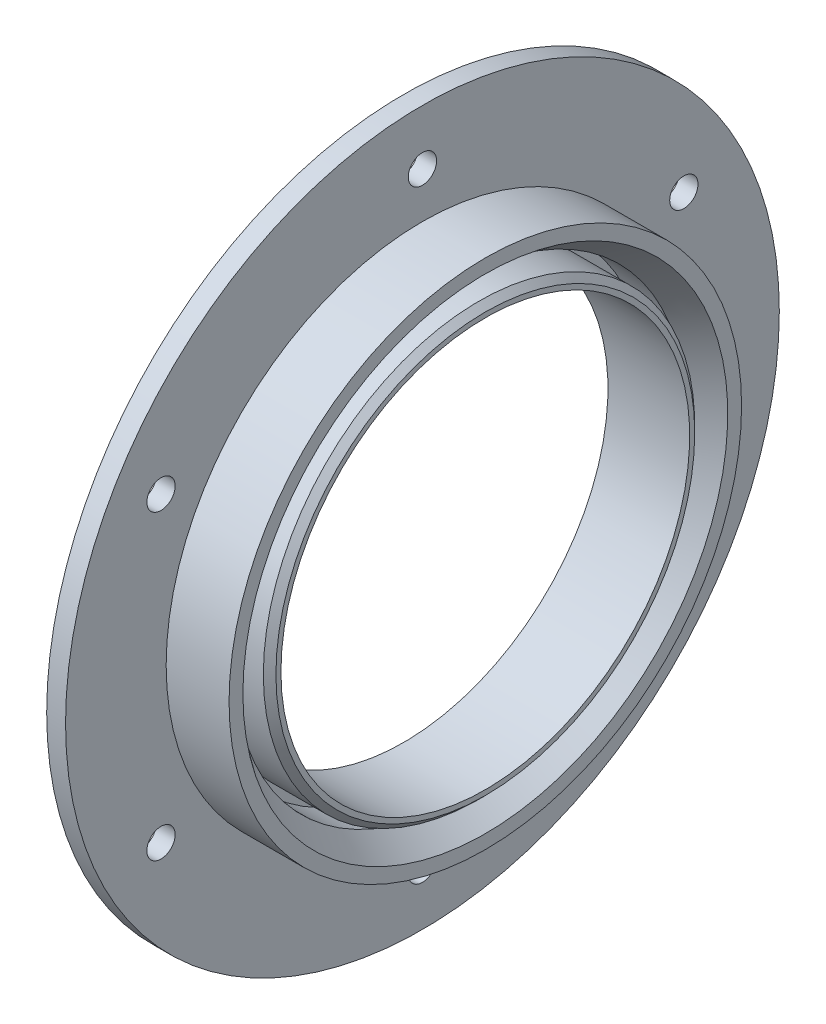
from build123d import *

# Parameters (mm, degrees)
CHAMFER1_SIZE      = 4
CHAMFER1_SIZE2     = 2.800830153
CHAMFER2_SIZE      = 1
SKETCH2_R          = 2.25
CUT_EXTRUDE1_DEPTH = 10
CIRPATTERN1_COUNT  = 6


with BuildPart() as part:
    # Sketch1 → Revolve1 (revolve)
    with BuildSketch(Plane.XY, mode=Mode.PRIVATE) as revolve1_sk:
        Polygon((0, 32.5), (13, 32.5), (13, 34.3), (3, 34.3), (3, 35.75), (13, 35.75), (13, 40.75), (3, 40.75), (3, 56.75), (0, 56.75), align=None)
    revolve(revolve1_sk.sketch.rotate(Axis((0, 0, 0), (1, 0, 0)), 90), axis=Axis((0, 0, 0), (1, 0, 0)))

    # Chamfer1
    chamfer1_edges = [part.edges().sort_by_distance(p)[0] for p in [
        (13, 0, -35.75),
    ]]
    chamfer1_side = [part.faces().sort_by_distance(p)[0] for p in [
        (8, 0, -35.75),
    ]]
    chamfer(chamfer1_edges, length=CHAMFER1_SIZE, length2=CHAMFER1_SIZE2, reference=chamfer1_side[0])

    # Chamfer2
    chamfer2_edges = [part.edges().sort_by_distance(p)[0] for p in [
        (13, 0, -34.3),
    ]]
    chamfer(chamfer2_edges, length=CHAMFER2_SIZE)

    # Sketch2 → Cut-Extrude1 (cut)
    with BuildSketch(Plane(origin=(3, 0, 0), x_dir=(0, 0, -1), z_dir=(1, 0, 0))):
        with Locations((0, 48)):
            Circle(SKETCH2_R)
    cut_extrude1 = extrude(amount=-CUT_EXTRUDE1_DEPTH, mode=Mode.SUBTRACT)

    # CirPattern1: Cut-Extrude1 ×6 about axis
    cirpattern1_axis = Axis((0, 0, 0), (1, 0, 0))
    for i in range(1, CIRPATTERN1_COUNT):
        add(cut_extrude1.rotate(cirpattern1_axis, i * 360 / CIRPATTERN1_COUNT), mode=Mode.SUBTRACT)


solid = part.part
